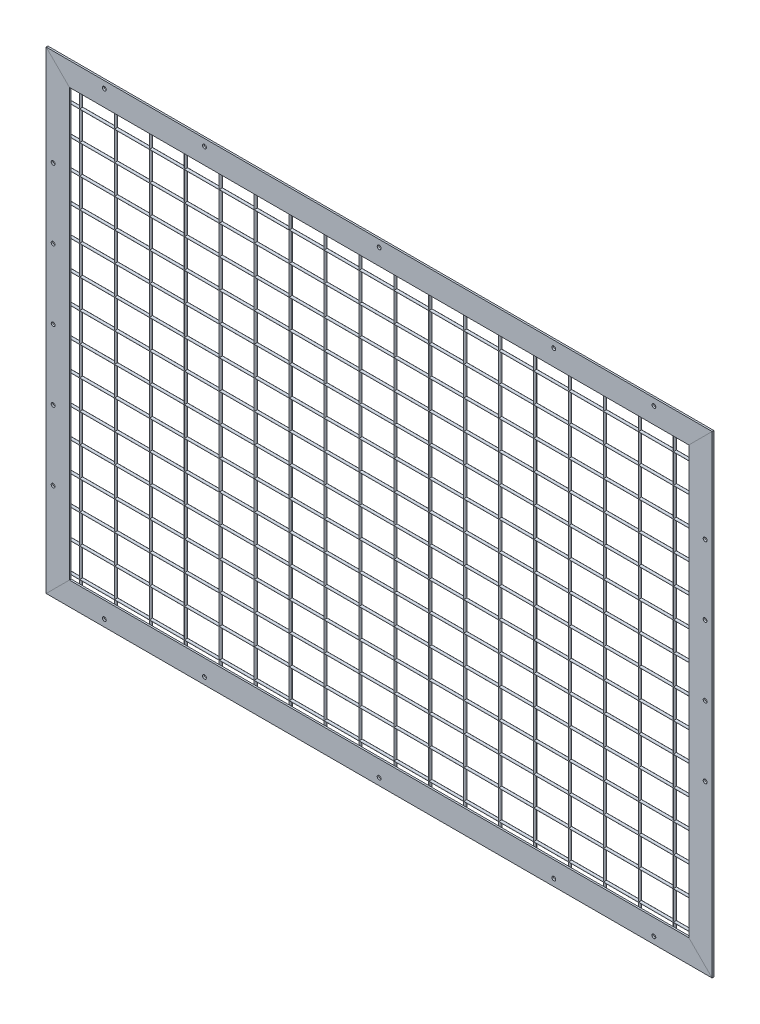
from build123d import *

# Parameters (mm, degrees)
EXTRUDE_2_DEPTH              = 3
EXTRUDE_2_2_DEPTH            = 3
EXTRUDE_3_DEPTH              = 3
EXTRUDE_3_2_DEPTH            = 3
SKETCH_7_R                   = 2
EXTRUDE_4_DEPTH              = 763
EXTRUDE_4_2_DEPTH            = 763
EXTRUDE_4_3_DEPTH            = 763
EXTRUDE_4_4_DEPTH            = 763
EXTRUDE_4_5_DEPTH            = 763
EXTRUDE_4_6_DEPTH            = 763
EXTRUDE_4_7_DEPTH            = 763
EXTRUDE_4_8_DEPTH            = 763
EXTRUDE_4_9_DEPTH            = 763
EXTRUDE_4_10_DEPTH           = 763
EXTRUDE_4_11_DEPTH           = 763
EXTRUDE_4_12_DEPTH           = 763
EXTRUDE_4_13_DEPTH           = 763
EXTRUDE_4_14_DEPTH           = 763
EXTRUDE_4_15_DEPTH           = 763
EXTRUDE_4_16_DEPTH           = 763
EXTRUDE_4_17_DEPTH           = 763
EXTRUDE_4_18_DEPTH           = 763
SKETCH_8_R                   = 2
EXTRUDE_5_DEPTH              = 1094
SKETCH_9_W                   = 3.3
SKETCH_9_H                   = 3.001
HOLE_WIZARD_M6_1_AT_2_COUNT  = 2
HOLE_WIZARD_M6_1_AT_2_PITCH  = 472
HOLE_WIZARD_M6_1_AT_3_COUNT  = 2
HOLE_WIZARD_M6_1_AT_3_PITCH  = 177.803965085
HOLE_WIZARD_M6_1_AT_4_COUNT  = 2
HOLE_WIZARD_M6_1_AT_4_PITCH  = 640.573375969
HOLE_WIZARD_M6_1_AT_5_COUNT  = 2
HOLE_WIZARD_M6_1_AT_5_PITCH  = 1230.307685093
HOLE_WIZARD_M6_1_AT_6_COUNT  = 2
HOLE_WIZARD_M6_1_AT_6_PITCH  = 919.404698705
HOLE_WIZARD_M6_1_AT_7_COUNT  = 2
HOLE_WIZARD_M6_1_AT_7_PITCH  = 789
HOLE_WIZARD_M6_1_AT_8_COUNT  = 2
HOLE_WIZARD_M6_1_AT_8_PITCH  = 172
HOLE_WIZARD_M6_1_AT_9_COUNT  = 2
HOLE_WIZARD_M6_1_AT_9_PITCH  = 807.530185194
HOLE_WIZARD_M6_1_AT_10_COUNT = 2
HOLE_WIZARD_M6_1_AT_10_PITCH = 1103.859139564
HOLE_WIZARD_M6_1_AT_11_COUNT = 2
HOLE_WIZARD_M6_1_AT_11_PITCH = 288.260732671
HOLE_WIZARD_M6_1_AT_12_COUNT = 2
HOLE_WIZARD_M6_1_AT_12_PITCH = 404.19580651
HOLE_WIZARD_M6_1_AT_13_COUNT = 2
HOLE_WIZARD_M6_1_AT_13_PITCH = 521.971503054
HOLE_WIZARD_M6_1_AT_14_COUNT = 2
HOLE_WIZARD_M6_1_AT_14_PITCH = 1067.883069442
HOLE_WIZARD_M6_1_AT_15_COUNT = 2
HOLE_WIZARD_M6_1_AT_15_PITCH = 1104.832227082
HOLE_WIZARD_M6_1_AT_16_COUNT = 2
HOLE_WIZARD_M6_1_AT_16_PITCH = 1153.141036474
HOLE_WIZARD_M6_1_AT_17_COUNT = 2
HOLE_WIZARD_M6_1_AT_17_PITCH = 772
HOLE_WIZARD_M6_1_AT_18_COUNT = 2
HOLE_WIZARD_M6_1_AT_18_PITCH = 944
HOLE_WIZARD_M6_1_AT_19_COUNT = 2
HOLE_WIZARD_M6_1_AT_19_PITCH = 1043.500958313


with BuildPart() as part:
    # 草图4 → 凸台-拉伸2 (new body)
    with BuildSketch(Plane.XY):
        Polygon((0, 0), (40, 40), (40, 773), (0, 813), align=None)
    extrude(amount=EXTRUDE_2_DEPTH)


with BuildPart() as body_2:
    # 草图4 → Extrude 2 2 (new body)
    with BuildSketch(Plane.XY):
        Polygon((1104, 40), (1144, 0), (1144, 813), (1104, 773), align=None)
    extrude(amount=EXTRUDE_2_2_DEPTH)


with BuildPart() as body_3:
    # 草图6 → 凸台-拉伸3 (new body)
    with BuildSketch(Plane.XY.offset(3)):
        Polygon((0, 0), (1144, 0), (1104, 40), (40, 40), align=None)
    extrude(amount=-EXTRUDE_3_DEPTH)


with BuildPart() as body_4:
    # 草图6 → Extrude 3 2 (new body)
    with BuildSketch(Plane.XY.offset(3)):
        Polygon((0, 813), (1144, 813), (1104, 773), (40, 773), align=None)
    extrude(amount=-EXTRUDE_3_2_DEPTH)

    # 草图9 → M6 间隙孔1 (revolve, cut)
    with BuildSketch(Plane(origin=(100, 801, 3), x_dir=(0, -1, 0), z_dir=(1, 0, 0))):
        with Locations((1.65, 1.5005)):
            Rectangle(SKETCH_9_W, SKETCH_9_H)
    hole_wizard_m6_1 = revolve(axis=Axis((100, 801, 9.35), (0, 0, -1)), mode=Mode.SUBTRACT)

    # M6 间隙孔1 at 2: M6 间隙孔1 ×2
    with Locations(*[(i * HOLE_WIZARD_M6_1_AT_2_PITCH, 0, 0) for i in range(1, HOLE_WIZARD_M6_1_AT_2_COUNT)]):
        add(hole_wizard_m6_1, mode=Mode.SUBTRACT)

    # M6 间隙孔1 at 8: M6 间隙孔1 ×2
    with Locations(*[(i * HOLE_WIZARD_M6_1_AT_8_PITCH, 0, 0) for i in range(1, HOLE_WIZARD_M6_1_AT_8_COUNT)]):
        add(hole_wizard_m6_1, mode=Mode.SUBTRACT)

    # M6 间隙孔1 at 17: M6 间隙孔1 ×2
    with Locations(*[(i * HOLE_WIZARD_M6_1_AT_17_PITCH, 0, 0) for i in range(1, HOLE_WIZARD_M6_1_AT_17_COUNT)]):
        add(hole_wizard_m6_1, mode=Mode.SUBTRACT)

    # M6 间隙孔1 at 18: M6 间隙孔1 ×2
    with Locations(*[(i * HOLE_WIZARD_M6_1_AT_18_PITCH, 0, 0) for i in range(1, HOLE_WIZARD_M6_1_AT_18_COUNT)]):
        add(hole_wizard_m6_1, mode=Mode.SUBTRACT)


with BuildPart() as body_5:
    # 草图7 → 凸台-拉伸4 (new body)
    with BuildSketch(Plane(origin=(0, 25, 0), x_dir=(-1, 0, 0), z_dir=(0, -1, 0))):
        with Locations(Location((-55, 2, 0), (0, 0, 90))):
            Circle(SKETCH_7_R)
    extrude(amount=-EXTRUDE_4_DEPTH)



with BuildPart() as body_6:
    # 草图7 → Extrude 4 2 (new body)
    with BuildSketch(Plane(origin=(0, 25, 0), x_dir=(-1, 0, 0), z_dir=(0, -1, 0))):
        with Locations(Location((-115, 2, 0), (0, 0, 90))):
            Circle(SKETCH_7_R)
    extrude(amount=-EXTRUDE_4_2_DEPTH)


with BuildPart() as body_7:
    # 草图7 → Extrude 4 3 (new body)
    with BuildSketch(Plane(origin=(0, 25, 0), x_dir=(-1, 0, 0), z_dir=(0, -1, 0))):
        with Locations(Location((-175, 2, 0), (0, 0, 90))):
            Circle(SKETCH_7_R)
    extrude(amount=-EXTRUDE_4_3_DEPTH)


with BuildPart() as body_8:
    # 草图7 → Extrude 4 4 (new body)
    with BuildSketch(Plane(origin=(0, 25, 0), x_dir=(-1, 0, 0), z_dir=(0, -1, 0))):
        with Locations(Location((-235, 2, 0), (0, 0, 90))):
            Circle(SKETCH_7_R)
    extrude(amount=-EXTRUDE_4_4_DEPTH)


with BuildPart() as body_9:
    # 草图7 → Extrude 4 5 (new body)
    with BuildSketch(Plane(origin=(0, 25, 0), x_dir=(-1, 0, 0), z_dir=(0, -1, 0))):
        with Locations(Location((-295, 2, 0), (0, 0, 90))):
            Circle(SKETCH_7_R)
    extrude(amount=-EXTRUDE_4_5_DEPTH)


with BuildPart() as body_10:
    # 草图7 → Extrude 4 6 (new body)
    with BuildSketch(Plane(origin=(0, 25, 0), x_dir=(-1, 0, 0), z_dir=(0, -1, 0))):
        with Locations(Location((-355, 2, 0), (0, 0, 90))):
            Circle(SKETCH_7_R)
    extrude(amount=-EXTRUDE_4_6_DEPTH)


with BuildPart() as body_11:
    # 草图7 → Extrude 4 7 (new body)
    with BuildSketch(Plane(origin=(0, 25, 0), x_dir=(-1, 0, 0), z_dir=(0, -1, 0))):
        with Locations(Location((-415, 2, 0), (0, 0, 90))):
            Circle(SKETCH_7_R)
    extrude(amount=-EXTRUDE_4_7_DEPTH)


with BuildPart() as body_12:
    # 草图7 → Extrude 4 8 (new body)
    with BuildSketch(Plane(origin=(0, 25, 0), x_dir=(-1, 0, 0), z_dir=(0, -1, 0))):
        with Locations(Location((-475, 2, 0), (0, 0, 90))):
            Circle(SKETCH_7_R)
    extrude(amount=-EXTRUDE_4_8_DEPTH)


with BuildPart() as body_13:
    # 草图7 → Extrude 4 9 (new body)
    with BuildSketch(Plane(origin=(0, 25, 0), x_dir=(-1, 0, 0), z_dir=(0, -1, 0))):
        with Locations(Location((-535, 2, 0), (0, 0, 90))):
            Circle(SKETCH_7_R)
    extrude(amount=-EXTRUDE_4_9_DEPTH)


with BuildPart() as body_14:
    # 草图7 → Extrude 4 10 (new body)
    with BuildSketch(Plane(origin=(0, 25, 0), x_dir=(-1, 0, 0), z_dir=(0, -1, 0))):
        with Locations(Location((-595, 2, 0), (0, 0, 90))):
            Circle(SKETCH_7_R)
    extrude(amount=-EXTRUDE_4_10_DEPTH)


with BuildPart() as body_15:
    # 草图7 → Extrude 4 11 (new body)
    with BuildSketch(Plane(origin=(0, 25, 0), x_dir=(-1, 0, 0), z_dir=(0, -1, 0))):
        with Locations(Location((-655, 2, 0), (0, 0, 90))):
            Circle(SKETCH_7_R)
    extrude(amount=-EXTRUDE_4_11_DEPTH)


with BuildPart() as body_16:
    # 草图7 → Extrude 4 12 (new body)
    with BuildSketch(Plane(origin=(0, 25, 0), x_dir=(-1, 0, 0), z_dir=(0, -1, 0))):
        with Locations(Location((-715, 2, 0), (0, 0, 90))):
            Circle(SKETCH_7_R)
    extrude(amount=-EXTRUDE_4_12_DEPTH)


with BuildPart() as body_17:
    # 草图7 → Extrude 4 13 (new body)
    with BuildSketch(Plane(origin=(0, 25, 0), x_dir=(-1, 0, 0), z_dir=(0, -1, 0))):
        with Locations(Location((-775, 2, 0), (0, 0, 90))):
            Circle(SKETCH_7_R)
    extrude(amount=-EXTRUDE_4_13_DEPTH)


with BuildPart() as body_18:
    # 草图7 → Extrude 4 14 (new body)
    with BuildSketch(Plane(origin=(0, 25, 0), x_dir=(-1, 0, 0), z_dir=(0, -1, 0))):
        with Locations(Location((-835, 2, 0), (0, 0, 90))):
            Circle(SKETCH_7_R)
    extrude(amount=-EXTRUDE_4_14_DEPTH)


with BuildPart() as body_19:
    # 草图7 → Extrude 4 15 (new body)
    with BuildSketch(Plane(origin=(0, 25, 0), x_dir=(-1, 0, 0), z_dir=(0, -1, 0))):
        with Locations(Location((-895, 2, 0), (0, 0, 90))):
            Circle(SKETCH_7_R)
    extrude(amount=-EXTRUDE_4_15_DEPTH)


with BuildPart() as body_20:
    # 草图7 → Extrude 4 16 (new body)
    with BuildSketch(Plane(origin=(0, 25, 0), x_dir=(-1, 0, 0), z_dir=(0, -1, 0))):
        with Locations(Location((-955, 2, 0), (0, 0, 90))):
            Circle(SKETCH_7_R)
    extrude(amount=-EXTRUDE_4_16_DEPTH)


with BuildPart() as body_21:
    # 草图7 → Extrude 4 17 (new body)
    with BuildSketch(Plane(origin=(0, 25, 0), x_dir=(-1, 0, 0), z_dir=(0, -1, 0))):
        with Locations(Location((-1015, 2, 0), (0, 0, 90))):
            Circle(SKETCH_7_R)
    extrude(amount=-EXTRUDE_4_17_DEPTH)


with BuildPart() as body_22:
    # 草图7 → Extrude 4 18 (new body)
    with BuildSketch(Plane(origin=(0, 25, 0), x_dir=(-1, 0, 0), z_dir=(0, -1, 0))):
        with Locations(Location((-1075, 2, 0), (0, 0, 90))):
            Circle(SKETCH_7_R)
    extrude(amount=-EXTRUDE_4_18_DEPTH)


with BuildPart() as body_5_1:
    add(body_5.part)

    add(body_6.part)  # 凸台-拉伸5 merges body 6

    add(body_7.part)  # 凸台-拉伸5 merges body 7

    add(body_8.part)  # 凸台-拉伸5 merges body 8

    add(body_9.part)  # 凸台-拉伸5 merges body 9

    add(body_10.part)  # 凸台-拉伸5 merges body 10

    add(body_11.part)  # 凸台-拉伸5 merges body 11

    add(body_12.part)  # 凸台-拉伸5 merges body 12

    add(body_13.part)  # 凸台-拉伸5 merges body 13

    add(body_14.part)  # 凸台-拉伸5 merges body 14

    add(body_15.part)  # 凸台-拉伸5 merges body 15

    add(body_16.part)  # 凸台-拉伸5 merges body 16

    add(body_17.part)  # 凸台-拉伸5 merges body 17

    add(body_18.part)  # 凸台-拉伸5 merges body 18

    add(body_19.part)  # 凸台-拉伸5 merges body 19

    add(body_20.part)  # 凸台-拉伸5 merges body 20

    add(body_21.part)  # 凸台-拉伸5 merges body 21

    add(body_22.part)  # 凸台-拉伸5 merges body 22
    # 草图8 → 凸台-拉伸5 (add)
    with BuildSketch(Plane.ZY.offset(-25)):
        with Locations((-2, 47.1)):
            Circle(SKETCH_8_R)
        with Locations((-2, 97.1)):
            Circle(SKETCH_8_R)
        with Locations((-2, 147.1)):
            Circle(SKETCH_8_R)
        with Locations((-2, 197.1)):
            Circle(SKETCH_8_R)
        with Locations((-2, 247.1)):
            Circle(SKETCH_8_R)
        with Locations((-2, 297.1)):
            Circle(SKETCH_8_R)
        with Locations((-2, 347.1)):
            Circle(SKETCH_8_R)
        with Locations((-2, 397.1)):
            Circle(SKETCH_8_R)
        with Locations((-2, 447.1)):
            Circle(SKETCH_8_R)
        with Locations((-2, 497.1)):
            Circle(SKETCH_8_R)
        with Locations((-2, 547.1)):
            Circle(SKETCH_8_R)
        with Locations((-2, 597.1)):
            Circle(SKETCH_8_R)
        with Locations((-2, 647.1)):
            Circle(SKETCH_8_R)
        with Locations((-2, 697.1)):
            Circle(SKETCH_8_R)
        with Locations((-2, 747.1)):
            Circle(SKETCH_8_R)
    extrude(amount=-EXTRUDE_5_DEPTH)


with BuildPart() as part_1:
    add(part.part)

    # M6 间隙孔1 at 3: M6 间隙孔1 ×2
    with Locations(*[Vector(-0.494927095455147, -0.8689345028161396, 0) * (i * HOLE_WIZARD_M6_1_AT_3_PITCH) for i in range(1, HOLE_WIZARD_M6_1_AT_3_COUNT)]):
        add(hole_wizard_m6_1, mode=Mode.SUBTRACT)

    # M6 间隙孔1 at 4: M6 间隙孔1 ×2
    with Locations(*[Vector(-0.137376924020478, -0.9905188442158341, 0) * (i * HOLE_WIZARD_M6_1_AT_4_PITCH) for i in range(1, HOLE_WIZARD_M6_1_AT_4_COUNT)]):
        add(hole_wizard_m6_1, mode=Mode.SUBTRACT)

    # M6 间隙孔1 at 11: M6 间隙孔1 ×2
    with Locations(*[Vector(-0.3052791796670006, -0.9522628956658152, 0) * (i * HOLE_WIZARD_M6_1_AT_11_PITCH) for i in range(1, HOLE_WIZARD_M6_1_AT_11_COUNT)]):
        add(hole_wizard_m6_1, mode=Mode.SUBTRACT)

    # M6 间隙孔1 at 12: M6 间隙孔1 ×2
    with Locations(*[Vector(-0.21771626172943806, -0.9760121051393568, 0) * (i * HOLE_WIZARD_M6_1_AT_12_PITCH) for i in range(1, HOLE_WIZARD_M6_1_AT_12_COUNT)]):
        add(hole_wizard_m6_1, mode=Mode.SUBTRACT)

    # M6 间隙孔1 at 13: M6 间隙孔1 ×2
    with Locations(*[Vector(-0.16859157920536694, -0.9856859943313796, 0) * (i * HOLE_WIZARD_M6_1_AT_13_PITCH) for i in range(1, HOLE_WIZARD_M6_1_AT_13_COUNT)]):
        add(hole_wizard_m6_1, mode=Mode.SUBTRACT)


with BuildPart() as body_3_1:
    add(body_3.part)

    # M6 间隙孔1 at 5: M6 间隙孔1 ×2
    with Locations(*[Vector(0.7672877373990379, -0.6413029923811874, 0) * (i * HOLE_WIZARD_M6_1_AT_5_PITCH) for i in range(1, HOLE_WIZARD_M6_1_AT_5_COUNT)]):
        add(hole_wizard_m6_1, mode=Mode.SUBTRACT)

    # M6 间隙孔1 at 6: M6 间隙孔1 ×2
    with Locations(*[Vector(0.5133756665210151, -0.8581639849260184, 0) * (i * HOLE_WIZARD_M6_1_AT_6_PITCH) for i in range(1, HOLE_WIZARD_M6_1_AT_6_COUNT)]):
        add(hole_wizard_m6_1, mode=Mode.SUBTRACT)

    # M6 间隙孔1 at 7: M6 间隙孔1 ×2
    with Locations(*[(0, -i * HOLE_WIZARD_M6_1_AT_7_PITCH, 0) for i in range(1, HOLE_WIZARD_M6_1_AT_7_COUNT)]):
        add(hole_wizard_m6_1, mode=Mode.SUBTRACT)

    # M6 间隙孔1 at 9: M6 间隙孔1 ×2
    with Locations(*[Vector(0.2129951339944121, -0.9770532600092497, 0) * (i * HOLE_WIZARD_M6_1_AT_9_PITCH) for i in range(1, HOLE_WIZARD_M6_1_AT_9_COUNT)]):
        add(hole_wizard_m6_1, mode=Mode.SUBTRACT)

    # M6 间隙孔1 at 10: M6 间隙孔1 ×2
    with Locations(*[Vector(0.6993645949288404, -0.7147651106202786, 0) * (i * HOLE_WIZARD_M6_1_AT_10_PITCH) for i in range(1, HOLE_WIZARD_M6_1_AT_10_COUNT)]):
        add(hole_wizard_m6_1, mode=Mode.SUBTRACT)


with BuildPart() as body_2_1:
    add(body_2.part)

    # M6 间隙孔1 at 14: M6 间隙孔1 ×2
    with Locations(*[Vector(0.9663979414334593, -0.25705061523593464, 0) * (i * HOLE_WIZARD_M6_1_AT_14_PITCH) for i in range(1, HOLE_WIZARD_M6_1_AT_14_COUNT)]):
        add(hole_wizard_m6_1, mode=Mode.SUBTRACT)

    # M6 间隙孔1 at 15: M6 间隙孔1 ×2
    with Locations(*[Vector(0.9340784733671342, -0.3570677885109829, 0) * (i * HOLE_WIZARD_M6_1_AT_15_PITCH) for i in range(1, HOLE_WIZARD_M6_1_AT_15_COUNT)]):
        add(hole_wizard_m6_1, mode=Mode.SUBTRACT)

    # M6 间隙孔1 at 16: M6 间隙孔1 ×2
    with Locations(*[Vector(0.8949469035944738, -0.4461726568792217, 0) * (i * HOLE_WIZARD_M6_1_AT_16_PITCH) for i in range(1, HOLE_WIZARD_M6_1_AT_16_COUNT)]):
        add(hole_wizard_m6_1, mode=Mode.SUBTRACT)

    # M6 间隙孔1 at 19: M6 间隙孔1 ×2
    with Locations(*[Vector(0.9889784880202482, -0.1480592794565197, 0) * (i * HOLE_WIZARD_M6_1_AT_19_PITCH) for i in range(1, HOLE_WIZARD_M6_1_AT_19_COUNT)]):
        add(hole_wizard_m6_1, mode=Mode.SUBTRACT)


solid = Compound([body_4.part, body_5_1.part, part_1.part, body_3_1.part, body_2_1.part])
